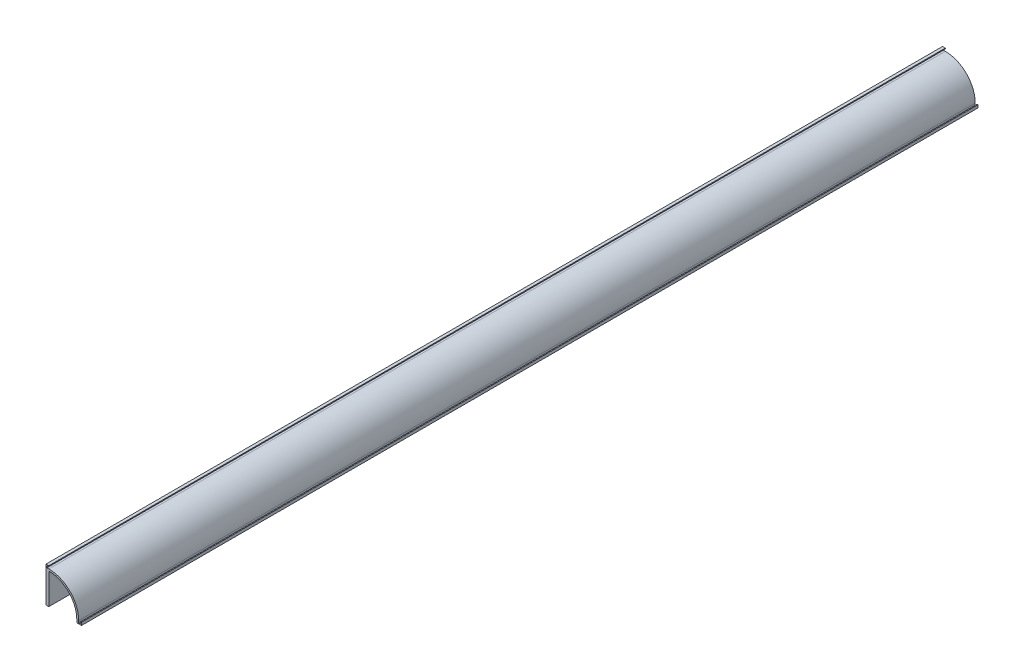
from build123d import *

# Parameters (mm, degrees)
BOSS_EXTRUDE1_DEPTH = 480


with BuildPart() as part:
    # Sketch1 → Boss-Extrude1 (new body)
    with BuildSketch(Plane.XY):
        with BuildLine():
            Line((0, 0), (0, 19))
            Line((0, 19), (1.5, 19))
            Line((1.5, 19), (1.5, 18.5))
            Line((1.5, 18.5), (0.5, 18.5))
            Line((0.5, 18.5), (0.5, 17.5))
            Line((0.5, 17.5), (1.5, 17.5))
            ThreePointArc((1.5, 17.5), (12.813708499, 12.813708499), (17.5, 1.5))
            Line((17.5, 1.5), (17.5, 0.5))
            Line((17.5, 0.5), (18.5, 0.5))
            Line((18.5, 0.5), (18.5, 1.5))
            Line((18.5, 1.5), (19, 1.5))
            Line((19, 1.5), (19, 0))
            Line((19, 0), (16.5, 0))
            Line((16.5, 0), (16.5, 1.5))
            ThreePointArc((16.5, 1.5), (12.106601718, 12.106601718), (1.5, 16.5))
            Line((1.5, 16.5), (1.5, 0))
            Line((1.5, 0), (0, 0))
        make_face()
    extrude(amount=BOSS_EXTRUDE1_DEPTH)


solid = part.part
